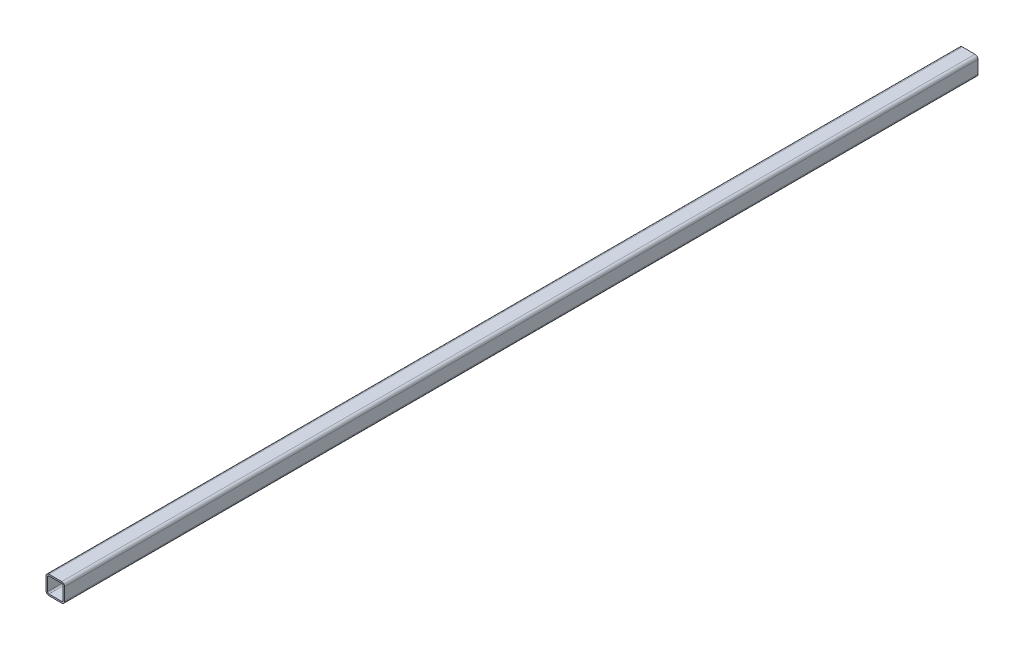
SolidWorks part; units mm, degrees
material "Q235"
ref_plane "Plane1" through (0, 0, 0) normal (0, 0, 1) x (1, 0, 0)
ref_plane "Plane2" through (0, 0, 0) normal (0, 1, 0) x (1, 0, 0)
ref_plane "Plane3" through (0, 0, 0) normal (1, 0, 0) x (0, 0, -1)
sketch "Sketch1" plane through (0, 0, 0) normal (0, 0, 1) x (1, 0, 0)
  line L0 (-8.5, -10.5) -> (8.5, -10.5)
  line L1 (-10.5, -8.5) -> (-10.5, 8.5)
  line L2 (8.5, 10.5) -> (-8.5, 10.5)
  line L3 (10.5, 8.5) -> (10.5, -8.5)
  line L4 (-8.5, -12.5) -> (8.5, -12.5)
  line L5 (-12.5, -8.5) -> (-12.5, 8.5)
  line L6 (8.5, 12.5) -> (-8.5, 12.5)
  line L7 (12.5, 8.5) -> (12.5, -8.5)
  arc A0 (12.5, 8.5) -> (8.5, 12.5) centre (8.5, 8.5) ccw
  arc A1 (8.5, -12.5) -> (12.5, -8.5) centre (8.5, -8.5) ccw
  arc A2 (-12.5, -8.5) -> (-8.5, -12.5) centre (-8.5, -8.5) ccw
  arc A3 (-8.5, 12.5) -> (-12.5, 8.5) centre (-8.5, 8.5) ccw
  arc A4 (-8.5, 10.5) -> (-10.5, 8.5) centre (-8.5, 8.5) ccw
  arc A5 (10.5, 8.5) -> (8.5, 10.5) centre (8.5, 8.5) ccw
  arc A6 (8.5, -10.5) -> (10.5, -8.5) centre (8.5, -8.5) ccw
  arc A7 (-10.5, -8.5) -> (-8.5, -10.5) centre (-8.5, -8.5) ccw
  point P0 (0, 12.5)
  point P1 (12.5, 0)
  point P2 (0, -12.5)
  point P3 (-12.5, 0)
  point P4 (-12.5, 12.5)
  point P5 (12.5, 12.5)
  point P6 (12.5, -12.5)
  point P7 (-12.5, -12.5)
  point P8 (0, 0)
extrude "Boss-Extrude1" add sketch "Sketch1" along normal blind 1224
